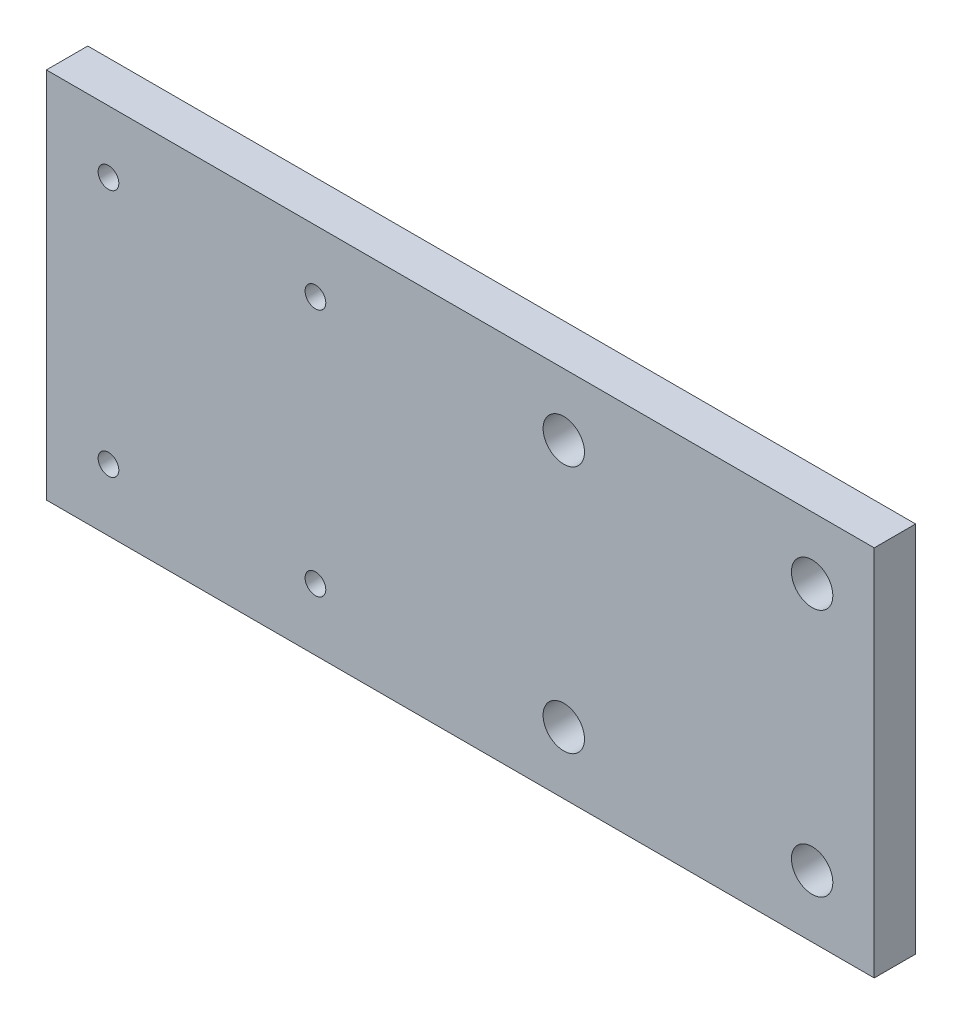
from build123d import *

# Parameters (mm, degrees)
SKETCH_1_W             = 200
SKETCH_1_H             = 90
EXTRUDE_1_DEPTH        = 10
HOLE_WIZARD_M6_1_D     = 5
HOLE_WIZARD_M8_1_D     = 10
HOLE_WIZARD_M8_1_DEPTH = 30
HOLE_WIZARD_M8_1_TIP   = 3.004303095


with BuildPart() as part:
    # 草图1 → 凸台-拉伸1 (new body)
    with BuildSketch(Plane.XY):
        Rectangle(SKETCH_1_W, SKETCH_1_H)
    extrude(amount=EXTRUDE_1_DEPTH)

    # M6 螺纹孔1 (through all)
    with Locations(Plane(origin=(0, 0, 0), x_dir=(-1, 0, 0), z_dir=(0, 0, -1))):
        with Locations((85, 30), (35, -30), (85, -30), (35, 30)):
            Hole(HOLE_WIZARD_M6_1_D / 2)

    # M8 间隙孔1
    with Locations(Plane.XY.offset(10)):
        with Locations((85, -30), (85, 30), (25, -30), (25, 30)):
            Hole(HOLE_WIZARD_M8_1_D / 2, depth=HOLE_WIZARD_M8_1_DEPTH)
            with Locations((0, 0, -(HOLE_WIZARD_M8_1_DEPTH + HOLE_WIZARD_M8_1_TIP / 2))):  # 118° drill point
                Cone(0, HOLE_WIZARD_M8_1_D / 2, HOLE_WIZARD_M8_1_TIP, mode=Mode.SUBTRACT)


solid = part.part
